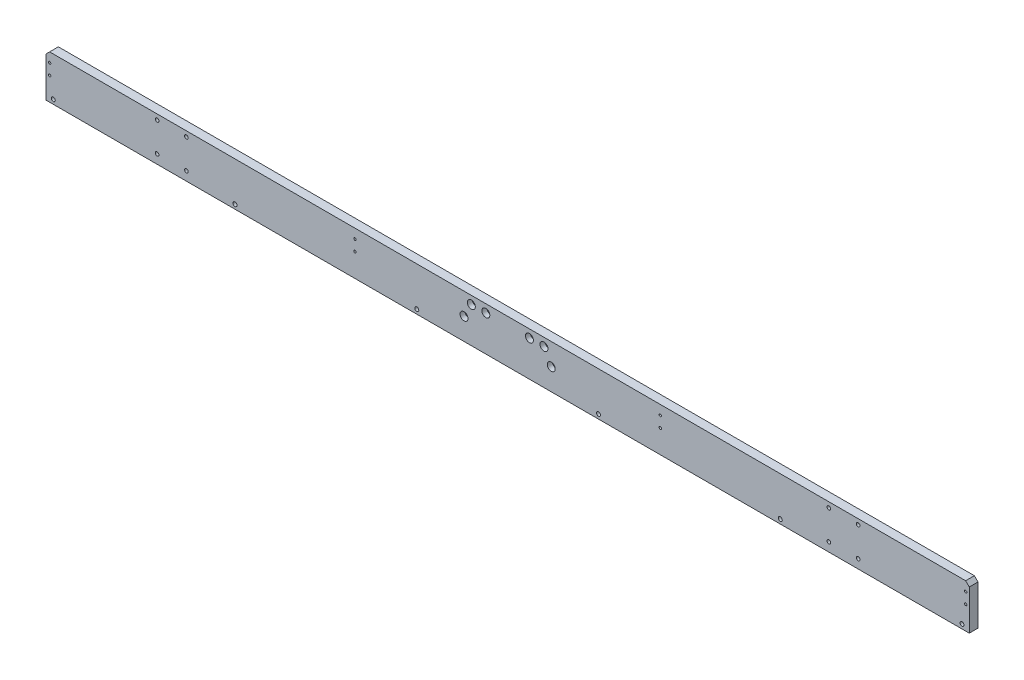
SolidWorks part; units mm, degrees
material "A6061"
ref_plane "前视基准面" through (0, 0, 0) normal (0, 0, 1) x (1, 0, 0)
ref_plane "上视基准面" through (0, 0, 0) normal (0, 1, 0) x (1, 0, 0)
ref_plane "右视基准面" through (0, 0, 0) normal (1, 0, 0) x (0, 0, -1)
sketch "草图1" plane through (0, 0, 0) normal (0, 0, 1) x (1, 0, 0)
  line L1 (-635, -30) -> (635, -30)
  line L2 (-635, -30) -> (-635, 30)
  line L3 (-635, 30) -> (635, 30)
  line L4 (635, -30) -> (635, 30)
  line L5 (-635, -30) -> (635, 30) construction
  line L6 (-635, 30) -> (635, -30) construction
  point P0 (0, 0)
  dimension "D1" = 1270
  dimension "D2" = 60
extrude "凸台-拉伸1" add sketch "草图1" along normal blind 12
chamfer "倒角1" distance 5 angle 45 2 edges at (-635, 30, 6) (635, 30, 6)
hole_wizard "打孔尺寸(%根据)内六角圆柱头螺钉的类型1" positions "草图2" profile "草图3" counterbore size "M5" standard "GB" end condition through all
sketch "草图2" plane through (0, 0, 0) normal (0, 0, -1) x (-1, 0, 0)
  line L0 (0, 0) -> (0, -63.2365) construction
  line L3 (635, -30) -> (-635, -30) construction
  point P0 (-625, -24)
  point P5 (-375, -24)
  point P6 (-125, -24)
  point P7 (125, -24)
  point P8 (375, -24)
  point P9 (625, -24)
  dimension "D2" = 250
  dimension "D3" = 6
  dimension "D1" = 6
sketch "草图3" plane through (625, -24, 0) normal (1, 0, 0) x (0, 1, 0)
  line L0 (0, 0) -> (0, 12)
  line L1 (0, 12) -> (2.75, 12)
  line L3 (2.75, 12) -> (2.75, 5.7)
  line L4 (2.75, 5.7) -> (5, 5.7)
  line L5 (5, 5.7) -> (5, 0)
  line L7 (5, 0) -> (0, 0)
  line L11 (0, -6.35) -> (0, 107.95) construction
  dimension "通孔孔直径" = 5.5
  dimension "通孔孔深度" = 12
  dimension "柱形沉头孔直径" = 10
  dimension "柱形沉头孔深度" = 5.7
hole_wizard "M6 螺纹孔1" positions "草图5" profile "草图6" tap size "M6" standard "GB" end condition through all
sketch "草图5" plane through (0, 0, 0) normal (0, 0, -1) x (-1, 0, 0)
  line L0 (0, 0) -> (0, 148.0802) construction
  line L2 (-630, 30) -> (630, 30) construction
  circle A0 centre (-462, 2.5) radius 28.5 construction
  circle A1 centre (462, 2.5) radius 28.5 construction
  point P0 (-482.1525, 22.6525)
  point P6 (-441.8475, 22.6525)
  point P7 (-441.8475, -17.6525)
  point P8 (-482.1525, -17.6525)
  point P23 (482.1525, -17.6525)
  point P24 (441.8475, -17.6525)
  point P25 (441.8475, 22.6525)
  point P26 (482.1525, 22.6525)
  dimension "D2" = 57
  dimension "D3" = 924
  dimension "D4" = 27.5
  dimension "D1" = 4
sketch "草图6" plane through (482.1525, 22.6525, 0) normal (1, 0, 0) x (0, 1, 0)
  line L0 (0, 0) -> (0, 12)
  line L1 (0, 12) -> (2.5, 12)
  line L2 (2.5, 12) -> (2.5, 0)
  line L5 (2.5, 0) -> (0, 0)
  line L11 (0, -6.35) -> (0, 107.95) construction
  dimension "通孔螺纹孔钻头直径" = 5
  dimension "通孔螺纹孔钻头深度" = 12
cosmetic thread "孔螺蚊线27"
cosmetic thread "孔螺蚊线28"
cosmetic thread "孔螺蚊线29"
cosmetic thread "孔螺蚊线30"
cosmetic thread "孔螺蚊线31"
cosmetic thread "孔螺蚊线32"
cosmetic thread "孔螺蚊线33"
cosmetic thread "孔螺蚊线34"
hole_wizard "M4 螺纹孔1" positions "草图7" profile "草图8" tap size "M4" standard "GB" end condition through all
sketch "草图7" plane through (0, 0, 12) normal (0, 0, 1) x (1, 0, 0)
  line L0 (0, 0) -> (0, 112.0465) construction
  line L2 (-635, 25) -> (-635, -30) construction
  line L3 (630, 30) -> (-630, 30) construction
  point P0 (-630, 17)
  point P2 (-630, 2)
  point P8 (630, 2)
  point P9 (630, 17)
  point P14 (-210, 17)
  point P16 (-210, 2)
  point P19 (210, 2)
  point P20 (210, 17)
  dimension "D1" = 5
  dimension "D2" = 15
  dimension "D3" = 13
  dimension "D4" = 420
sketch "草图8" plane through (-630, 17, 12) normal (1, 0, 0) x (0, -1, 0)
  line L0 (0, 0) -> (0, 12)
  line L1 (0, 12) -> (1.65, 12)
  line L2 (1.65, 12) -> (1.65, 0)
  line L5 (1.65, 0) -> (0, 0)
  line L11 (0, -6.35) -> (0, 107.95) construction
  dimension "通孔螺纹孔钻头直径" = 3.3
  dimension "通孔螺纹孔钻头深度" = 12
cosmetic thread "孔螺蚊线35"
cosmetic thread "孔螺蚊线36"
cosmetic thread "孔螺蚊线37"
cosmetic thread "孔螺蚊线38"
cosmetic thread "孔螺蚊线39"
cosmetic thread "孔螺蚊线40"
cosmetic thread "孔螺蚊线41"
cosmetic thread "孔螺蚊线42"
hole_wizard "打孔尺寸(%根据)内六角圆柱头螺钉的类型2" positions "草图9" profile "草图10" counterbore size "M6" standard "GB" end condition through all
sketch "草图9" plane through (0, 0, 12) normal (0, 0, 1) x (1, 0, 0)
  line L0 (0, 0) -> (0, 95.0268) construction
  line L2 (630, 30) -> (-630, 30) construction
  point P0 (-60, 0)
  point P2 (-50, 19)
  point P4 (-30, 19)
  point P12 (30, 19)
  point P13 (50, 19)
  point P14 (60, 0)
  dimension "D1" = 20
  dimension "D2" = 60
  dimension "D3" = 11
  dimension "D4" = 19
  dimension "D5" = 120
sketch "草图10" plane through (-60, 0, 12) normal (1, 0, 0) x (0, -1, 0)
  line L0 (0, 0) -> (0, 12)
  line L1 (0, 12) -> (3.3, 12)
  line L3 (3.3, 12) -> (3.3, 6.8)
  line L4 (3.3, 6.8) -> (5.5, 6.8)
  line L5 (5.5, 6.8) -> (5.5, 0)
  line L7 (5.5, 0) -> (0, 0)
  line L11 (0, -6.35) -> (0, 107.95) construction
  dimension "通孔孔直径" = 6.6
  dimension "通孔孔深度" = 12
  dimension "柱形沉头孔直径" = 11
  dimension "柱形沉头孔深度" = 6.8
